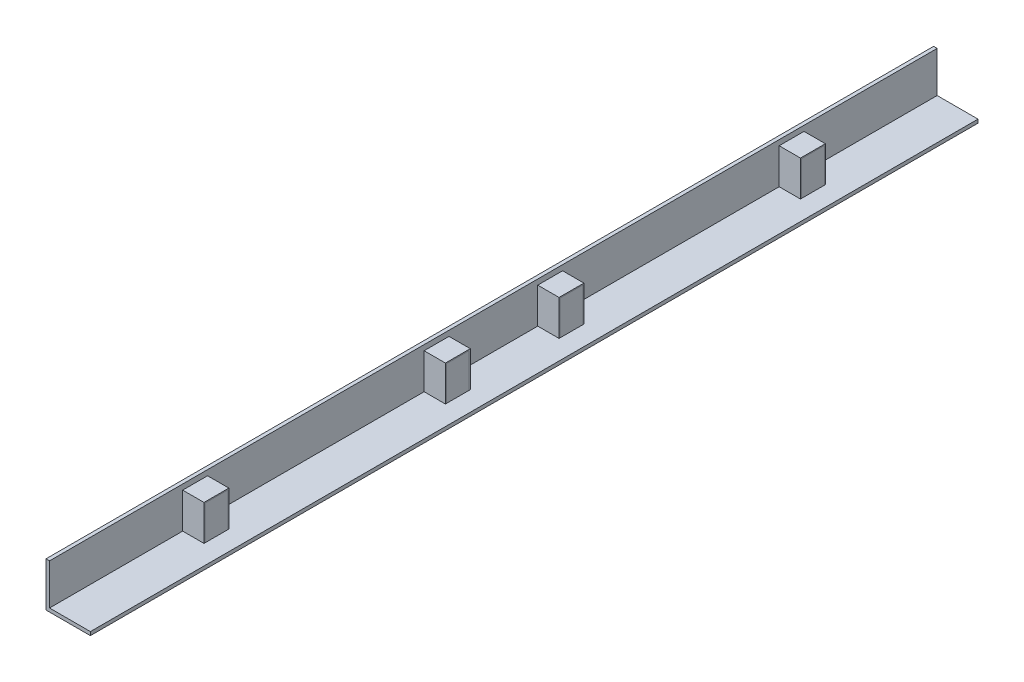
SolidWorks part; units mm, degrees
material "A3"
ref_plane "前视基准面" through (0, 0, 0) normal (0, 0, 1) x (1, 0, 0)
ref_plane "上视基准面" through (0, 0, 0) normal (0, 1, 0) x (1, 0, 0)
ref_plane "右视基准面" through (0, 0, 0) normal (1, 0, 0) x (0, 0, -1)
sketch "草图1" plane through (0, 0, 0) normal (0, 0, 1) x (1, 0, 0)
  line L0 (0, 125) -> (0, 0)
  line L1 (0, 0) -> (125, 0)
  line L2 (125, 0) -> (125, 10)
  line L3 (10, 125) -> (10, 10)
  line L4 (10, 10) -> (125, 10)
  line L5 (0, 125) -> (10, 125)
  dimension "D1" = 125
  dimension "D2" = 10
  dimension "D3" = 10
extrude "凸台-拉伸1" add sketch "草图1" along normal mid plane 2500 contours L5 L0 L1 L2 L4 L3
sketch "草图2" plane through (10, 0, 0) normal (1, 0, 0) x (0, 0, -1)
  line L0 (-872, 10) -> (-872, 107)
  line L1 (-1250, 10) -> (1250, 10) construction
  line L2 (-872, 107) -> (-808, 107)
  line L3 (-808, 107) -> (-808, 10)
  line L4 (-1250, 10) -> (1250, 10) construction
  point P5 (-840, 107)
  dimension "D1" = 97
  dimension "D2" = 64
  dimension "D3" = 840
extrude "拉伸-薄壁1" add sketch "草图2" along normal blind 60 separate body thin thin type one direction reverse wall 3
sketch "草图3" plane through (70, 0, 0) normal (1, 0, 0) x (0, 0, -1)
  line L1 (-872, 107) -> (-808, 107)
  line L2 (-872, 107) -> (-872, 10)
  line L3 (-872, 10) -> (-808, 10)
  line L4 (-808, 107) -> (-808, 10)
  line L5 (-1250, 10) -> (1250, 10) construction
  line L6 (-808, 107) -> (-808, 10) construction
extrude "凸台-拉伸2" add sketch "草图3" against normal blind 3 separate body
pattern_linear "阵列(线性)1" count 2 spacing 680 along (0, 0, -1) of bodies 117 118
mirror "镜向1" about plane through (0, 0, 0) normal (0, 0, 1) of bodies 120 117 119 118
sketch "草图4" plane through (0, 0, 0) normal (0, -1, 0) x (1, 0, 0)
  line L0 (0, 1250) -> (0, -1250) construction
  line L1 (67, 130) -> (21, 130)
  line L2 (67, 130) -> (67, 190)
  line L3 (67, 190) -> (21, 190)
  line L4 (21, 130) -> (21, 190)
  line L5 (67, 130) -> (21, 190) construction
  line L6 (67, 190) -> (21, 130) construction
  line L7 (0, 0) -> (125, 0) construction
  line L8 (21, 810) -> (67, 810)
  line L9 (21, 810) -> (21, 870)
  line L10 (21, 870) -> (67, 870)
  line L11 (67, 810) -> (67, 870)
  line L12 (21, 810) -> (67, 870) construction
  line L13 (21, 870) -> (67, 810) construction
  line L14 (125, 1250) -> (125, -1250) construction
  line L15 (21, -870) -> (67, -810) construction
  line L16 (21, -810) -> (67, -870) construction
  line L17 (67, -190) -> (21, -130) construction
  line L18 (67, -130) -> (21, -190) construction
  line L19 (67, -810) -> (67, -870)
  line L20 (21, -870) -> (67, -870)
  line L21 (21, -810) -> (21, -870)
  line L22 (21, -810) -> (67, -810)
  line L23 (21, -130) -> (21, -190)
  line L24 (67, -190) -> (21, -190)
  line L25 (67, -130) -> (67, -190)
  line L26 (67, -130) -> (21, -130)
  point P0 (44, 160)
  point P8 (44, 840)
  point P25 (44, -840)
  point P26 (44, -160)
  dimension "D1" = 60
  dimension "D2" = 21
  dimension "D3" = 160
  dimension "D4" = 60
  dimension "D5" = 840
  dimension "D6" = 46
  dimension "D7" = 46
extrude "切除-拉伸1" cut sketch "草图4" against normal blind 10
